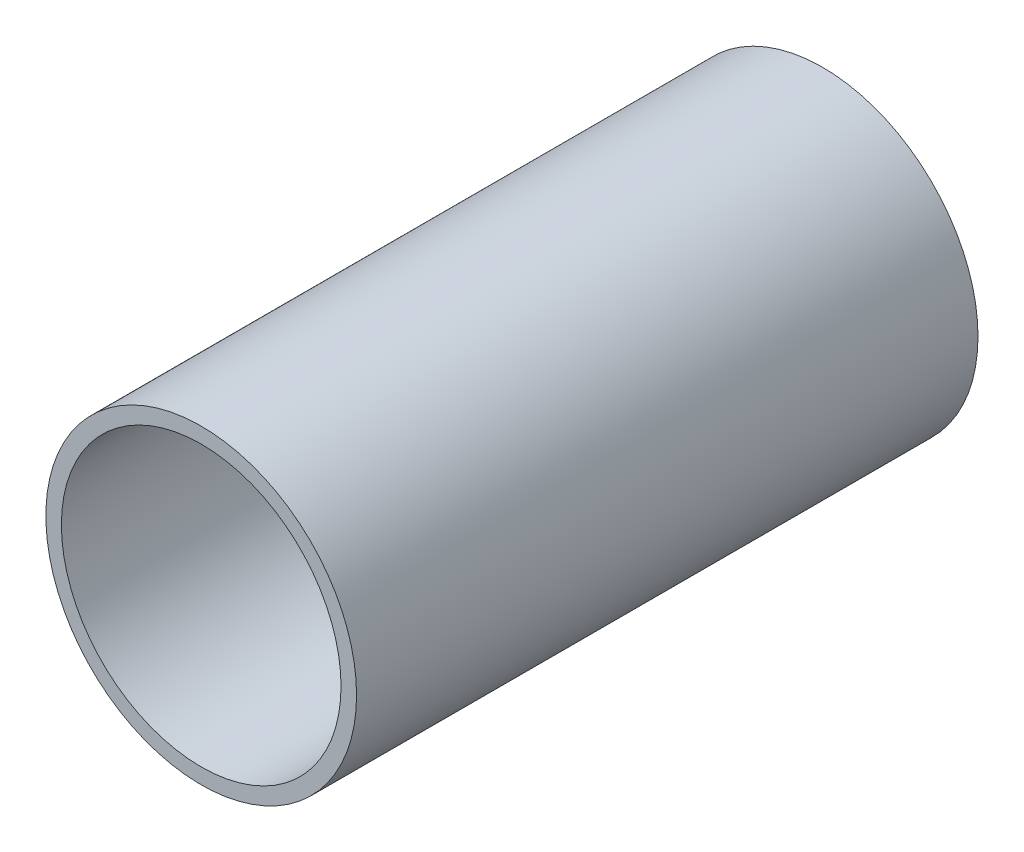
SolidWorks part; units mm, degrees
ref_plane "前视基准面" through (0, 0, 0) normal (0, 0, 1) x (1, 0, 0)
ref_plane "上视基准面" through (0, 0, 0) normal (0, 1, 0) x (1, 0, 0)
ref_plane "右视基准面" through (0, 0, 0) normal (1, 0, 0) x (0, 0, -1)
other "Configuration Table"
sketch "草图1" plane through (0, 0, 0) normal (0, 0, 1) x (1, 0, 0)
  circle A0 centre (0, 0) radius 20
  circle A1 centre (0, 0) radius 18
  point P0 (0, 0)
  dimension "D1" = 36
  dimension "D2" = 40
extrude "凸台-拉伸1" add sketch "草图1" against normal mid plane 80
